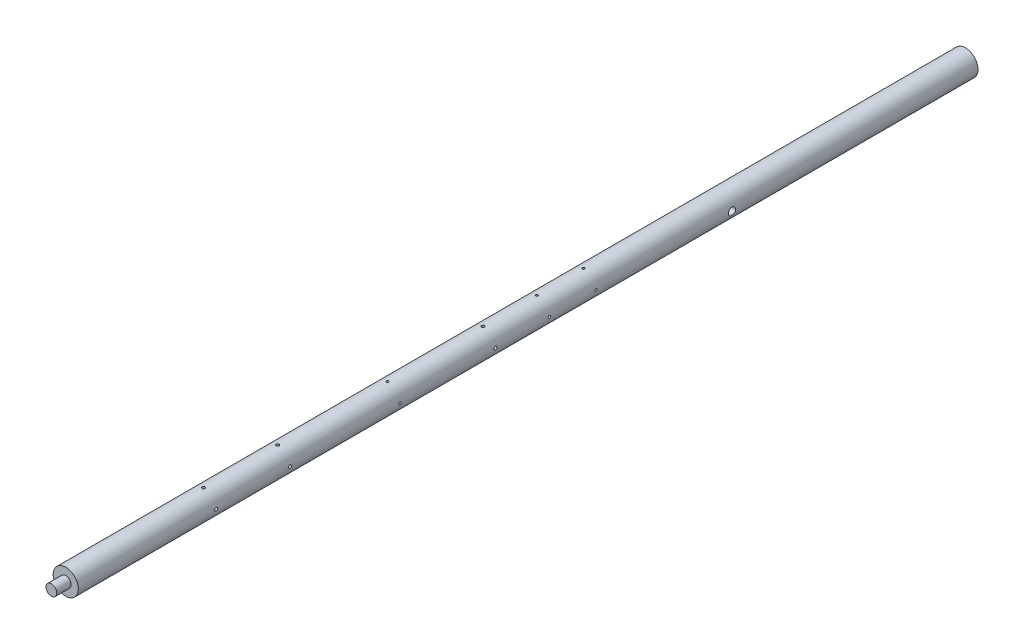
SolidWorks part; units mm, degrees
material "1.7005 (45Cr2)"
ref_plane "前视基准面" through (0, 0, 0) normal (0, 0, 1) x (1, 0, 0)
ref_plane "上视基准面" through (0, 0, 0) normal (0, 1, 0) x (1, 0, 0)
ref_plane "右视基准面" through (0, 0, 0) normal (1, 0, 0) x (0, 0, -1)
sketch "草图1" plane through (0, 0, 0) normal (0, 0, 1) x (1, 0, 0)
  circle A0 centre (0, 0) radius 17.5
  dimension "D1" = 35
extrude "凸台-拉伸1" add sketch "草图1" along normal blind 1313
sketch "草图2" plane through (0, 0, 1313) normal (0, 0, 1) x (1, 0, 0)
  circle A0 centre (0, 0) radius 7.5
  dimension "D1" = 15
extrude "凸台-拉伸2" add sketch "草图2" along normal blind 10
chamfer "倒角1" distance 1 angle 45 1 edges at (7.5, 0, 1323)
sketch "草图3" plane through (0, 0, 0) normal (1, 0, 0) x (0, 0, -1)
  line L0 (0, 0) -> (-312.5, 0) construction
  circle A0 centre (-312.5, 0) radius 5
  dimension "D1" = 10
  dimension "D2" = 312.5
extrude "切除-拉伸1" cut sketch "草图3" against normal mid plane 40
sketch "草图4" plane through (0, 0, 0) normal (0, 1, 0) x (1, 0, 0)
  line L0 (17.5, 0) -> (17.5, -502) construction
  line L1 (17.5, -307.5) -> (17.5, 0) construction
  dimension "D1" = 502
hole_wizard "M4x0.7 螺纹孔1" positions "3D草图1" profile "草图5" tap size "M4x0.7" standard "BSI"
sketch3d "3D草图1"
  point P0 (17.5, 0, 502)
sketch "草图5" plane through (17.5, 0, 502) normal (0, 1, 0) x (0, 0, -1)
  line L0 (0, 0) -> (0, 11.0914)
  line L1 (0, 11.0914) -> (1.65, 10.1)
  line L2 (1.65, 10.1) -> (1.65, 0)
  line L5 (1.65, 0) -> (0, 0)
  line L10 (0, 11.0914) -> (-1.65, 10.1) construction
  line L11 (0, -6.35) -> (0, 107.95) construction
  dimension "螺纹孔钻头直径" = 3.3
  dimension "螺纹孔钻头深度" = 10.1
  dimension "导头角度" = 118
cosmetic thread "孔螺蚊线1" parameters "D1"=8, "D2"=4
pattern_circular "阵列(圆周)1" count 4 over 360 about axis through (0, 0, 1313) along (0, 0, -1) of "M4x0.7 螺纹孔1"
cosmetic thread "孔螺蚊线2" parameters "D1"=8, "D2"=4
cosmetic thread "孔螺蚊线3" parameters "D1"=8, "D2"=4
cosmetic thread "孔螺蚊线4" parameters "D1"=8, "D2"=4
sketch "草图6" plane through (0, 0, 0) normal (0, 1, 0) x (1, 0, 0)
  line L0 (0, -1313) -> (0, 0) construction
  line L1 (-7.5, -1313) -> (7.5, -1313) construction
pattern_linear "阵列(线性)1" count 2 spacing 65 along (0, 0, 1) of "阵列(圆周)1", "M4x0.7 螺纹孔1"
cosmetic thread "孔螺蚊线5" parameters "D1"=8, "D2"=4
cosmetic thread "孔螺蚊线6" parameters "D1"=8, "D2"=4
cosmetic thread "孔螺蚊线7" parameters "D1"=8, "D2"=4
cosmetic thread "孔螺蚊线8" parameters "D1"=8, "D2"=4
sketch "草图7" plane through (0, 0, 0) normal (0, 1, 0) x (1, 0, 0)
  line L0 (17.5, 0) -> (17.5, -642) construction
  line L1 (17.5, -1313) -> (17.5, -568.65) construction
  dimension "D1" = 642
hole_wizard "M5x0.8 螺纹孔1" positions "3D草图2" profile "草图8" tap size "M5x0.8" standard "BSI"
sketch3d "3D草图2"
  point P0 (17.5, 0, 642)
sketch "草图8" plane through (17.5, 0, 642) normal (0, 1, 0) x (0, 0, -1)
  line L0 (0, 0) -> (0, 13.6618)
  line L1 (0, 13.6618) -> (2.1, 12.4)
  line L2 (2.1, 12.4) -> (2.1, 0)
  line L5 (2.1, 0) -> (0, 0)
  line L10 (0, 13.6618) -> (-2.1, 12.4) construction
  line L11 (0, -6.35) -> (0, 107.95) construction
  dimension "螺纹孔钻头直径" = 4.2
  dimension "螺纹孔钻头深度" = 12.4
  dimension "导头角度" = 118
cosmetic thread "孔螺蚊线9" parameters "D1"=10, "D2"=5
pattern_circular "阵列(圆周)2" count 4 over 360 about axis through (0, 0, 1313) along (0, 0, -1) of "M5x0.8 螺纹孔1"
cosmetic thread "孔螺蚊线10" parameters "D1"=10, "D2"=5
cosmetic thread "孔螺蚊线11" parameters "D1"=10, "D2"=5
cosmetic thread "孔螺蚊线12" parameters "D1"=10, "D2"=5
pattern_linear "阵列(线性)2" count 2 spacing 273 along (0, 0, 1) of "阵列(圆周)1", "M4x0.7 螺纹孔1"
cosmetic thread "孔螺蚊线13" parameters "D1"=8, "D2"=4
cosmetic thread "孔螺蚊线14" parameters "D1"=8, "D2"=4
cosmetic thread "孔螺蚊线15" parameters "D1"=8, "D2"=4
cosmetic thread "孔螺蚊线16" parameters "D1"=8, "D2"=4
pattern_linear "阵列(线性)3" count 2 spacing 286 along (0, 0, 1) of "阵列(圆周)2", "M5x0.8 螺纹孔1"
cosmetic thread "孔螺蚊线17" parameters "D1"=10, "D2"=5
cosmetic thread "孔螺蚊线18" parameters "D1"=10, "D2"=5
cosmetic thread "孔螺蚊线19" parameters "D1"=10, "D2"=5
cosmetic thread "孔螺蚊线20" parameters "D1"=10, "D2"=5
pattern_linear "阵列(线性)4" count 2 spacing 389 along (0, 0, 1) of "M5x0.8 螺纹孔1", "阵列(圆周)2"
cosmetic thread "孔螺蚊线21" parameters "D1"=10, "D2"=5
cosmetic thread "孔螺蚊线22" parameters "D1"=10, "D2"=5
cosmetic thread "孔螺蚊线23" parameters "D1"=10, "D2"=5
cosmetic thread "孔螺蚊线24" parameters "D1"=10, "D2"=5
sketch "草图9" plane through (0, 0, 1313) normal (0, 0, 1) x (1, 0, 0)
  circle A0 centre (0, 0) radius 7.5 construction
  circle A1 centre (0, 0) radius 17.5
  circle A2 centre (0, 0) radius 17.5
  circle A3 centre (0, 0) radius 7.5
  dimension "D1" = 0
extrude "切除-拉伸2" cut sketch "草图9" against normal blind 90
sketch "草图10" plane through (0, 0, 1323) normal (0, 0, 1) x (1, 0, 0)
  circle A0 centre (0, 0) radius 8.0934
extrude "切除-拉伸3" cut sketch "草图10" against normal blind 80
sketch "草图11" plane through (0, 0, 0) normal (0, 0, -1) x (-1, 0, 0)
  circle A1 centre (0, 0) radius 17.5
  circle A2 centre (0, 0) radius 17.5
  dimension "D1" = 0
extrude "凸台-拉伸3" add sketch "草图11" along normal blind 30
